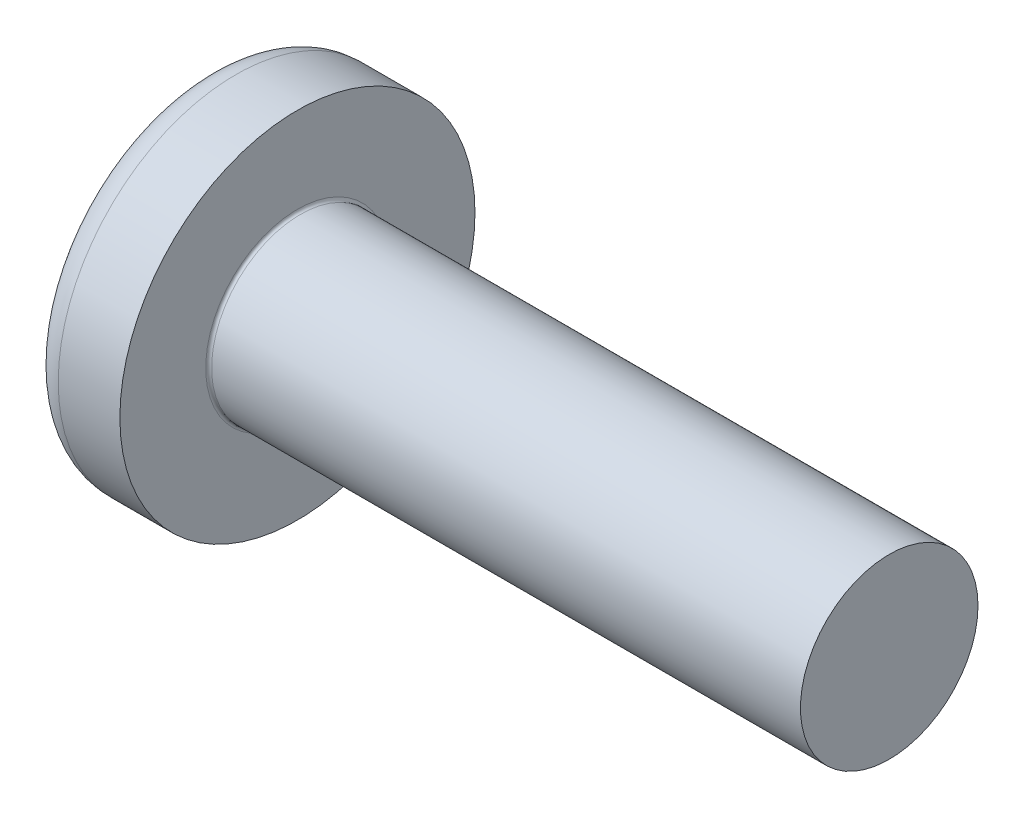
SolidWorks part; units mm, degrees
ref_plane "Front" through (0, 0, 0) normal (0, 0, 1) x (1, 0, 0)
ref_plane "Top" through (0, 0, 0) normal (0, 1, 0) x (1, 0, 0)
ref_plane "Right" through (0, 0, 0) normal (1, 0, 0) x (0, 0, -1)
other "Configuration Table"
sketch "Sketch1" plane through (0, 0, 0) normal (1, 0, 0) x (0, 0, -1)
  circle A0 centre (0, 0) radius 6
  dimension "dk" = 12
extrude "BaseHead" add sketch "Sketch1" along normal blind 4.6
sketch "Sketch2" plane through (4.6, 0, 0) normal (1, 0, 0) x (0, 0, -1)
  circle A0 centre (0, 0) radius 3
extrude "BaseBody" add sketch "Sketch2" along normal blind 20
cosmetic thread "ThreadCosmetic1" parameters "D1"=8, "THD_MINOR"=5
fillet "Fillet1" radius 0.1 1 edges at (4.6, 0, -3)
sketch "Sketch3" plane through (-4.0827, -1.9173, 0) normal (0, 0, 1) x (0, -1, 0)
  line L0 (-1.9173, 6.3195) -> (-1.9173, 20.448) construction
  line L3 (-7.9173, 4.0827) -> (-1.9173, 4.0827) construction
  line L5 (-7.9173, 6.0827) -> (-7.9173, -0.9173)
  line L6 (-1.9173, 4.0827) -> (-1.9173, -0.9173)
  line L7 (-1.9173, -0.9173) -> (-7.9173, -0.9173)
  line L8 (-7.9173, 8.6827) -> (-7.9173, 4.0827) construction
  arc A0 (-7.9173, 6.0827) -> (-1.9173, 4.0827) centre (-1.9173, 14.0827) ccw
  dimension "r1" = 10
  dimension "D2" = 5
revolve "BaseTop" cut sketch "Sketch3" angle 360 about L0
sketch "Sketch4" plane through (0, 0, 0) normal (1, 0, 0) x (0, 0, -1)
  line L1 (2.396, 0) -> (1.198, 2.075)
  line L2 (1.198, 2.075) -> (-1.198, 2.075)
  line L3 (-1.198, 2.075) -> (-2.396, 0)
  line L4 (-2.396, 0) -> (-1.198, -2.075)
  line L5 (-1.198, -2.075) -> (1.198, -2.075)
  line L6 (1.198, -2.075) -> (2.396, 0)
  circle A0 centre (0, 0) radius 2.075 construction
  dimension "B" = 4.15
extrude "Socket" cut sketch "Sketch4" along normal blind 2
sketch "Sketch5" plane through (2, 0, 0) normal (-1, 0, 0) x (0, 0, 1)
  line L0 (2.396, 0) -> (1.198, -2.075) construction
  line L1 (1.198, 2.075) -> (2.396, 0) construction
  line L2 (1.198, -2.075) -> (-1.198, -2.075) construction
  line L3 (-1.198, -2.075) -> (-2.396, 0) construction
  line L4 (-1.198, 2.075) -> (1.198, 2.075) construction
  line L5 (-2.396, 0) -> (-1.198, 2.075) construction
  line L6 (2.396, 0) -> (1.198, -2.075)
  line L7 (1.198, 2.075) -> (2.396, 0)
  line L8 (1.198, -2.075) -> (-1.198, -2.075)
  line L9 (-1.198, -2.075) -> (-2.396, 0)
  line L10 (-1.198, 2.075) -> (1.198, 2.075)
  line L11 (-2.396, 0) -> (-1.198, 2.075)
extrude "Cut-Extrude2" cut sketch "Sketch5" against normal blind 5 draft 60
sketch "Sketch6" plane through (-30.7487, 13.2487, 0) normal (0, 0, 1) x (0, -1, 0)
  line L0 (13.2487, 89.8637) -> (13.2487, 24.8312) construction
  line L1 (-4.2513, 35.3487) -> (10.6487, 35.3487)
  line L2 (-4.2513, 35.3487) -> (-4.2513, 45.3487)
  line L3 (-4.2513, 45.3487) -> (10.2487, 45.3487)
  line L4 (10.7487, 35.4487) -> (10.7487, 43.3487)
  line L5 (10.6487, 35.3487) -> (10.7487, 35.3487)
  line L6 (10.2487, 45.3487) -> (10.7487, 43.3487)
  line L7 (10.7487, 35.4487) -> (10.7487, 35.3487)
  line L8 (16.2487, 55.3487) -> (10.2487, 55.3487) construction
  line L9 (19.2487, 35.3487) -> (7.2487, 35.3487) construction
  arc A0 (10.6487, 35.3487) -> (10.7487, 35.4487) centre (10.6487, 35.4487) ccw construction
  dimension "d1" = 5
  dimension "D2" = 15
  dimension "b" = 10
  dimension "x" = 2
fillet "HeadFillet2" radius 1 1 edges at (2, 0, 6)
sketch "Sketch8" plane through (0, 0, 0) normal (0, 0, 1) x (1, 0, 0)
  line L0 (24.6, 2.567) -> (24.85, 3)
  line L1 (24.85, 3) -> (24.85, 3.5)
  line L2 (24.85, 3.5) -> (24.35, 3.5)
  line L3 (24.35, 3.5) -> (24.35, 3)
  line L4 (24.35, 3) -> (24.6, 2.567)
  line L5 (24.6, -3) -> (24.6, 3) construction
  line L6 (0, 0) -> (27.6816, 0) construction
revolve "Cut-Revolve10" [suppressed] cut sketch "Sketch8" angle 360 about L6
pattern_linear "LPattern10" [suppressed] count 13 spacing 0.6 along (1, 0, 0)
equation "\"D2@Sketch8\" = \"d@Sketch2\""
equation "\"D1@Sketch8\" =  ( \"d@Sketch2\" - \"THD_MINOR@ThreadCosmetic1\" )  / 2"
equation "\"D3@LPattern10\" = \"D1@Sketch8\" * 1.2"
equation "\"D1@LPattern10\" = \"D1@ThreadCosmetic1\" / \"D3@LPattern10\" "
